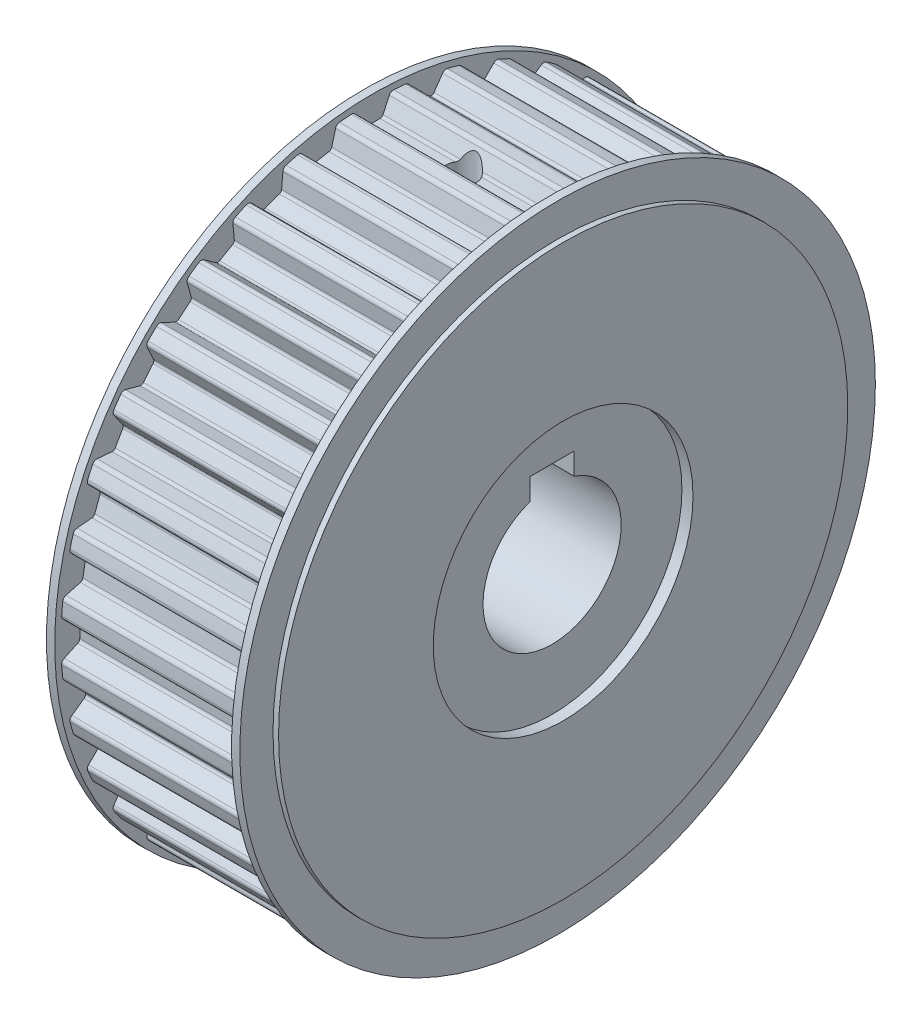
SolidWorks part; units mm, degrees
ref_plane "前视" through (0, 0, 0) normal (0, 0, 1) x (1, 0, 0)
ref_plane "上视" through (0, 0, 0) normal (0, 1, 0) x (1, 0, 0)
ref_plane "右视" through (0, 0, 0) normal (1, 0, 0) x (0, 0, -1)
sketch "草图1" plane through (0, 0, 0) normal (1, 0, 0) x (0, 0, -1)
  line L0 (0, 56.37) -> (0, 56.751) construction
  circle A1 centre (0, 0) radius 56.37
  circle A2 centre (0, 0) radius 56.751 construction
  dimension "D2" = 112.74
  dimension "D3" = 0.381
extrude "拉伸1" add sketch "草图1" along normal mid plane 32
sketch "草图2" plane through (16, 0, 0) normal (1, 0, 0) x (0, 0, -1)
  line L0 (0, 0) -> (0, 61.5267) construction
  line L1 (-3.285, 56.2742) -> (-1.7442, 52.97)
  line L2 (-1.7442, 52.97) -> (1.7442, 52.97)
  line L3 (1.7442, 52.97) -> (3.285, 56.2742)
  circle A0 centre (0, 0) radius 56.37 construction
  arc A1 (3.285, 56.2742) -> (-3.285, 56.2742) centre (0, 0) ccw
  dimension "D2" = 3.4
  dimension "D3" = 25
  dimension "D1" = 6.57
extrude "拉伸2" cut sketch "草图2" against normal up to surface (32 mm away) up to face at (-16, 0, -56.37)
fillet "圆角1" radius 0.6 2 edges at (0, 52.97, -1.7442) (0, 52.97, 1.7442)
fillet "圆角2" radius 0.8 2 edges at (0, 56.2742, -3.285) (0, 56.2742, 3.285)
pattern_circular "阵列(圆周)1" count 36 over 360 about axis through (0, 0, 0) along (1, 0, 0) of "拉伸2", "圆角1", "圆角2"
sketch "草图6" plane through (16, 0, 0) normal (1, 0, 0) x (0, 0, -1)
  circle A0 centre (0, 0) radius 57.5
  dimension "D1" = 115
extrude "凸台-拉伸2" add sketch "草图6" along normal blind 1.5
sketch "草图7" plane through (17.5, 0, 0) normal (1, 0, 0) x (0, 0, -1)
  circle A0 centre (0, 0) radius 51.5
  dimension "D1" = 103
extrude "凸台-拉伸3" add sketch "草图7" along normal blind 1
mirror "镜向2" about plane through (0, 0, 0) normal (1, 0, 0) of "凸台-拉伸3", "凸台-拉伸2"
sketch "草图8" plane through (-18.5, 0, 0) normal (-1, 0, 0) x (0, 0, 1)
  circle A0 centre (0, 0) radius 12.5
  dimension "D1" = 25
extrude "切除-拉伸1" cut sketch "草图8" against normal through all
sketch "草图11" plane through (0, 0, 0) normal (1, 0, 0) x (0, 0, -1)
  line L1 (-4, 15.8) -> (4, 15.8)
  line L2 (-4, 15.8) -> (-4, 6.7763)
  line L3 (-4, 6.7763) -> (4, 6.7763)
  line L4 (4, 15.8) -> (4, 6.7763)
  dimension "D1" = 8
  dimension "D2" = 4
  dimension "D3" = 15.8
extrude "切除-拉伸3" cut sketch "草图11" against normal mid plane 50
ref_plane "基准面2" through (0, 56.37, 0) normal (0, 1, 0) x (1, 0, 0)
hole_wizard "M4 螺纹孔1" positions "草图13" profile "草图12" tap size "M4" standard "ISO"
sketch "草图13" plane through (0, 56.37, 0) normal (0, -1, 0) x (-1, 0, 0)
  point P0 (0, 0)
sketch "草图12" plane through (0, 56.37, 0) normal (1, 0, 0) x (0, 0, 1)
  line L0 (0, 0) -> (0, 48.0914)
  line L1 (0, 48.0914) -> (1.65, 47.1)
  line L2 (1.65, 47.1) -> (1.65, 0)
  line L5 (1.65, 0) -> (0, 0)
  line L10 (0, 48.0914) -> (-1.65, 47.1) construction
  line L11 (0, -6.35) -> (0, 107.95) construction
  dimension "螺纹孔钻头直径" = 3.3
  dimension "螺纹孔钻头深度" = 47.1
  dimension "导头角度" = 118
cosmetic thread "孔螺蚊线3" parameters "D1"=40.57, "D2"=4
sketch "草图14" plane through (18.5, 0, 0) normal (1, 0, 0) x (0, 0, -1)
  circle A0 centre (0, 0) radius 23.5
  dimension "D1" = 47
extrude "切除-拉伸4" cut sketch "草图14" against normal blind 2
mirror "镜向3" about plane through (0, 0, 0) normal (1, 0, 0) of "切除-拉伸4"
hole_wizard "Ø5.5 (5.5) 直径孔1" positions "草图16" profile "草图15" hole size "Ø5.5" standard "ISO"
sketch "草图16" plane through (0, 56.37, 0) normal (0, 1, 0) x (1, 0, 0)
  point P0 (0, 0)
sketch "草图15" plane through (0, 56.37, 0) normal (1, 0, 0) x (0, 0, 1)
  line L0 (0, 0) -> (0, 36.6524)
  line L1 (0, 36.6524) -> (2.75, 35)
  line L2 (2.75, 35) -> (2.75, 0)
  line L5 (2.75, 0) -> (0, 0)
  line L10 (0, 36.6524) -> (-2.75, 35) construction
  line L11 (0, -6.35) -> (0, 107.95) construction
  dimension "孔直径" = 5.5
  dimension "孔深度" = 35
  dimension "导头角度" = 118
